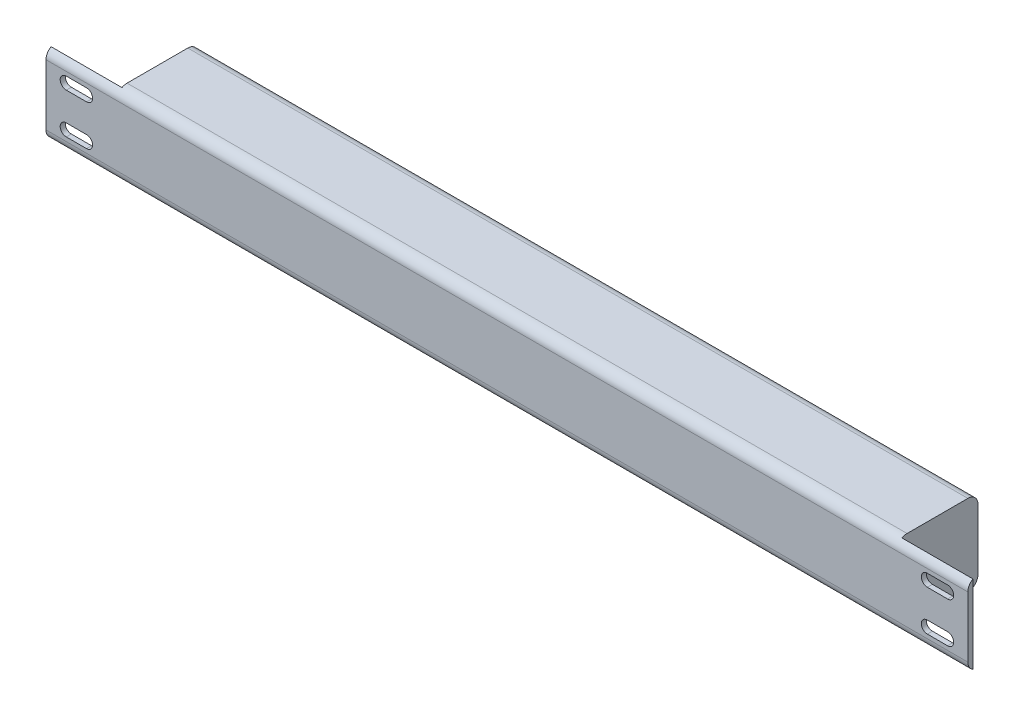
from build123d import *

# Parameters (mm, degrees)
SKETCH1_W           = 770
SKETCH1_H           = 80
BOSS_EXTRUDE1_DEPTH = 80
SKETCH3_W           = 5
SKETCH3_H           = 80
BOSS_EXTRUDE2_DEPTH = 70
SKETCH4_W           = 5
SKETCH4_H           = 80
BOSS_EXTRUDE3_DEPTH = 70
FILLET2_R           = 10
CUT_EXTRUDE1_DEPTH  = 690.814789958


with BuildPart() as part:
    # Sketch1 → Boss-Extrude1 (new body)
    with BuildSketch(Plane(origin=(0, 30, 0), x_dir=(1, 0, 0), z_dir=(0, 1, 0))):
        with Locations((228.333333333, 0)):
            Rectangle(SKETCH1_W, SKETCH1_H)
    extrude(amount=-BOSS_EXTRUDE1_DEPTH)

    # Sketch3 → Boss-Extrude2 (add)
    with BuildSketch(Plane.ZY.offset(156.666666667)):
        with Locations((37.5, -10)):
            Rectangle(SKETCH3_W, SKETCH3_H)
    extrude(amount=BOSS_EXTRUDE2_DEPTH)

    # Sketch4 → Boss-Extrude3 (add)
    with BuildSketch(Plane(origin=(613.333333333, 0, 0), x_dir=(0, 0, -1), z_dir=(1, 0, 0))):
        with Locations((-37.5, -10)):
            Rectangle(SKETCH4_W, SKETCH4_H)
    extrude(amount=BOSS_EXTRUDE3_DEPTH)

    # Fillet2
    fillet2_edges = [part.edges().sort_by_distance(p)[0] for p in [
        (228.333333333, 30, 40),
        (228.333333333, -50, 40),
        (228.333333333, -50, -40),
        (228.333333333, 30, -40),
    ]]
    fillet(fillet2_edges, radius=FILLET2_R)

    # Sketch6 → Cut-Extrude1 (cut, through all)
    with BuildSketch(Plane.XY.offset(40)):
        with BuildLine():
            Line((-206.666666667, -24), (-186.666666667, -24))
            ThreePointArc((-186.666666667, -24), (-180.666666667, -30), (-186.666666667, -36))
            Line((-186.666666667, -36), (-206.666666667, -36))
            ThreePointArc((-206.666666667, -36), (-212.666666667, -30), (-206.666666667, -24))
        make_face()
        with BuildLine():
            Line((-206.666666667, 16), (-186.666666667, 16))
            ThreePointArc((-186.666666667, 16), (-180.666666667, 10), (-186.666666667, 4))
            Line((-186.666666667, 4), (-206.666666667, 4))
            ThreePointArc((-206.666666667, 4), (-212.666666667, 10), (-206.666666667, 16))
        make_face()
        with BuildLine():
            Line((663.333333333, 16), (643.333333333, 16))
            ThreePointArc((643.333333333, 16), (637.333333333, 10), (643.333333333, 4))
            Line((643.333333333, 4), (663.333333333, 4))
            ThreePointArc((663.333333333, 4), (669.333333333, 10), (663.333333333, 16))
        make_face()
        with BuildLine():
            Line((663.333333333, -24), (643.333333333, -24))
            ThreePointArc((643.333333333, -24), (637.333333333, -30), (643.333333333, -36))
            Line((643.333333333, -36), (663.333333333, -36))
            ThreePointArc((663.333333333, -36), (669.333333333, -30), (663.333333333, -24))
        make_face()
    extrude(amount=-CUT_EXTRUDE1_DEPTH, mode=Mode.SUBTRACT)


solid = part.part
